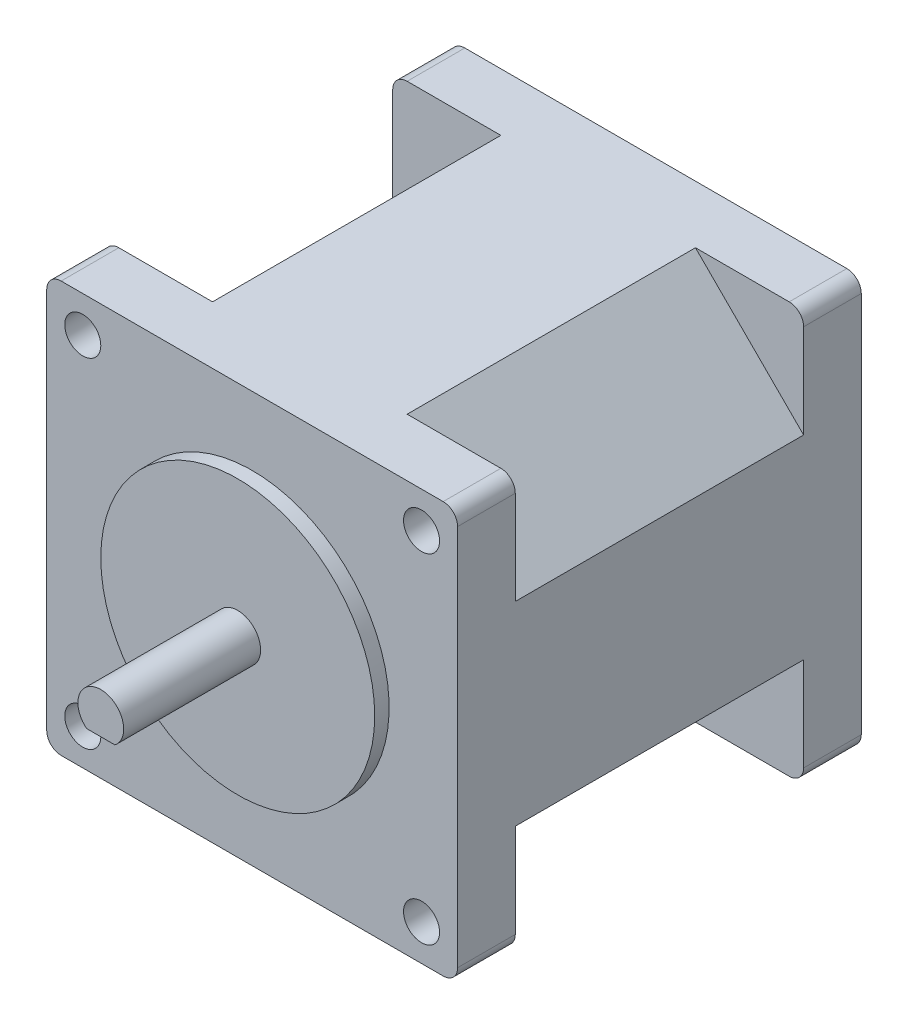
SolidWorks part; units mm, degrees
material "6061"
ref_plane "前视基准面" through (0, 0, 0) normal (0, 0, 1) x (1, 0, 0)
ref_plane "上视基准面" through (0, 0, 0) normal (0, 1, 0) x (1, 0, 0)
ref_plane "右视基准面" through (0, 0, 0) normal (1, 0, 0) x (0, 0, -1)
sketch "草图1" plane through (0, 0, 0) normal (0, 0, 1) x (1, 0, 0)
  line L1 (-28.5, -28.5) -> (28.5, -28.5)
  line L2 (-28.5, -28.5) -> (-28.5, 28.5)
  line L3 (-28.5, 28.5) -> (28.5, 28.5)
  line L4 (28.5, -28.5) -> (28.5, 28.5)
  line L5 (-28.5, -28.5) -> (28.5, 28.5) construction
  line L6 (-28.5, 28.5) -> (28.5, -28.5) construction
  point P0 (0, 0)
  dimension "D1" = 57
  dimension "D2" = 57
extrude "凸台-拉伸1" add sketch "草图1" along normal blind 56
sketch "草图2" plane through (0, 0, 56) normal (0, 0, 1) x (1, 0, 0)
  circle A0 centre (0, 0) radius 19
  dimension "D1" = 38
extrude "凸台-拉伸2" add sketch "草图2" along normal blind 2
sketch "草图3" plane through (0, 0, 58) normal (0, 0, 1) x (1, 0, 0)
  circle A0 centre (0, 0) radius 3.175
  dimension "D1" = 6.35
extrude "凸台-拉伸3" add sketch "草图3" along normal blind 19
ref_plane "基准面1" through (0, 0, 28) normal (0, 0, 1) x (1, 0, 0)
sketch "草图4" plane through (0, 0, 28) normal (0, 0, 1) x (1, 0, 0)
  line L0 (13.5, 28.5) -> (28.5, 13.5)
  line L1 (28.5, 28.5) -> (-28.5, 28.5) construction
  line L2 (28.5, -28.5) -> (28.5, 28.5) construction
  line L3 (28.5, 13.5) -> (28.5, 28.5)
  line L4 (28.5, 28.5) -> (13.5, 28.5)
  dimension "D1" = 15
  dimension "D2" = 15
extrude "切除-拉伸1" cut sketch "草图4" against normal mid plane 40
sketch "草图5" plane through (0, 0, 56) normal (0, 0, 1) x (1, 0, 0)
  circle A0 centre (23.5, 23.5) radius 2.5
  dimension "D1" = 5
  dimension "D2" = 23.5
  dimension "D3" = 23.5
extrude "切除-拉伸2" cut sketch "草图5" against normal up to surface (8 mm away) up to face at (23.5, 23.5, 48)
pattern_circular "阵列(圆周)1" count 4 over 360 about axis through (0, 0, 0) along (0, 0, 1) of "切除-拉伸1", "切除-拉伸2"
fillet "圆角1" radius 2 8 edges at (-28.5, 28.5, 4) (-28.5, 28.5, 52) (-28.5, -28.5, 4) (-28.5, -28.5, 52) (28.5, -28.5, 4) (28.5, -28.5, 52) (28.5, 28.5, 4) (28.5, 28.5, 52)
sketch "草图6" plane through (0, 0, 77) normal (0, 0, 1) x (1, 0, 0)
  line L1 (5.7449, -5.9672) -> (-5.6318, -5.9672)
  line L2 (5.7449, -5.9672) -> (5.7449, -2.5)
  line L3 (5.7449, -2.5) -> (-5.6318, -2.5)
  line L4 (-5.6318, -5.9672) -> (-5.6318, -2.5)
  dimension "D1" = 2.5
extrude "切除-拉伸3" cut sketch "草图6" against normal blind 15
